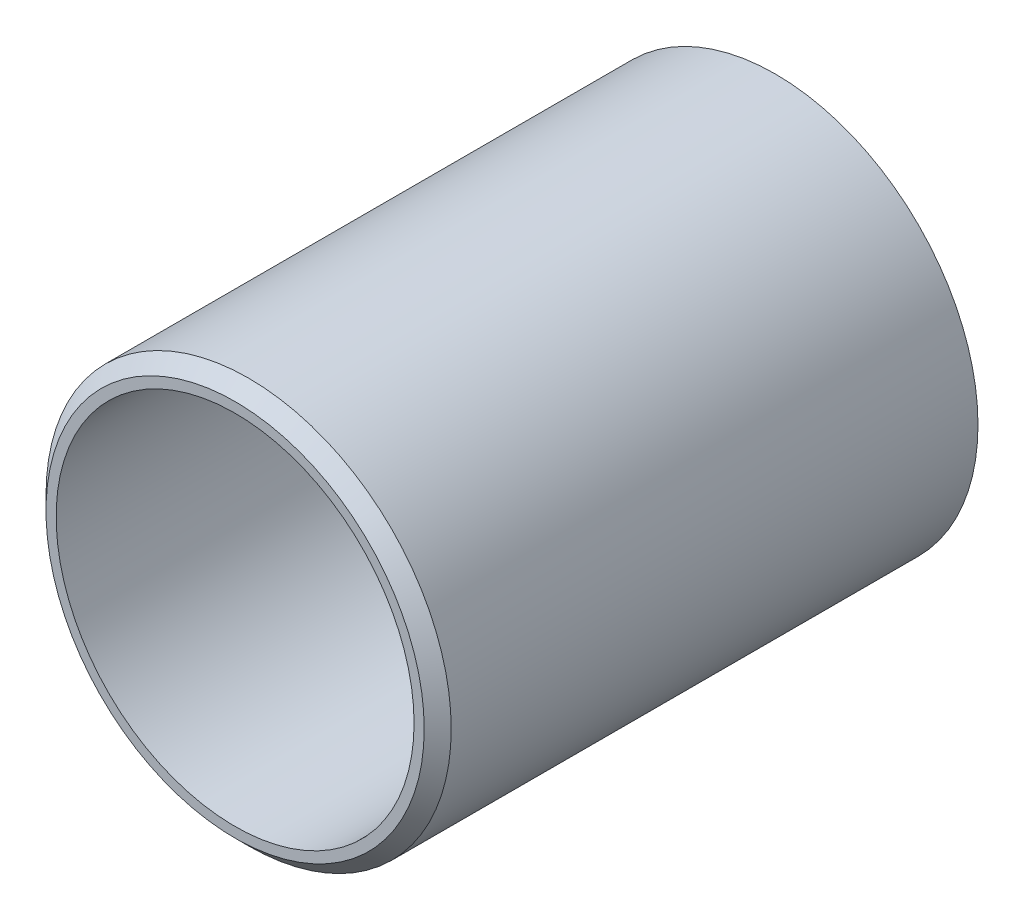
SolidWorks part; units mm, degrees
material "镀锌焊接钢管 Q215A"
ref_plane "前视基准面" through (0, 0, 0) normal (0, 0, 1) x (1, 0, 0)
ref_plane "上视基准面" through (0, 0, 0) normal (0, 1, 0) x (1, 0, 0)
ref_plane "右视基准面" through (0, 0, 0) normal (1, 0, 0) x (0, 0, -1)
sketch "草图1" plane through (0, 0, 0) normal (0, 0, 1) x (1, 0, 0)
  circle A0 centre (0, 0) radius 26.5
  circle A1 centre (0, 0) radius 30
  dimension "D1" = 60
  dimension "D2" = 3.5
extrude "拉伸1" add sketch "草图1" along normal blind 80
cosmetic thread "装饰螺纹线1" parameters "D1"=30, "D2"=56.656
chamfer "倒角1" distance 2 angle 45 1 edges at (30, 0, 80)
